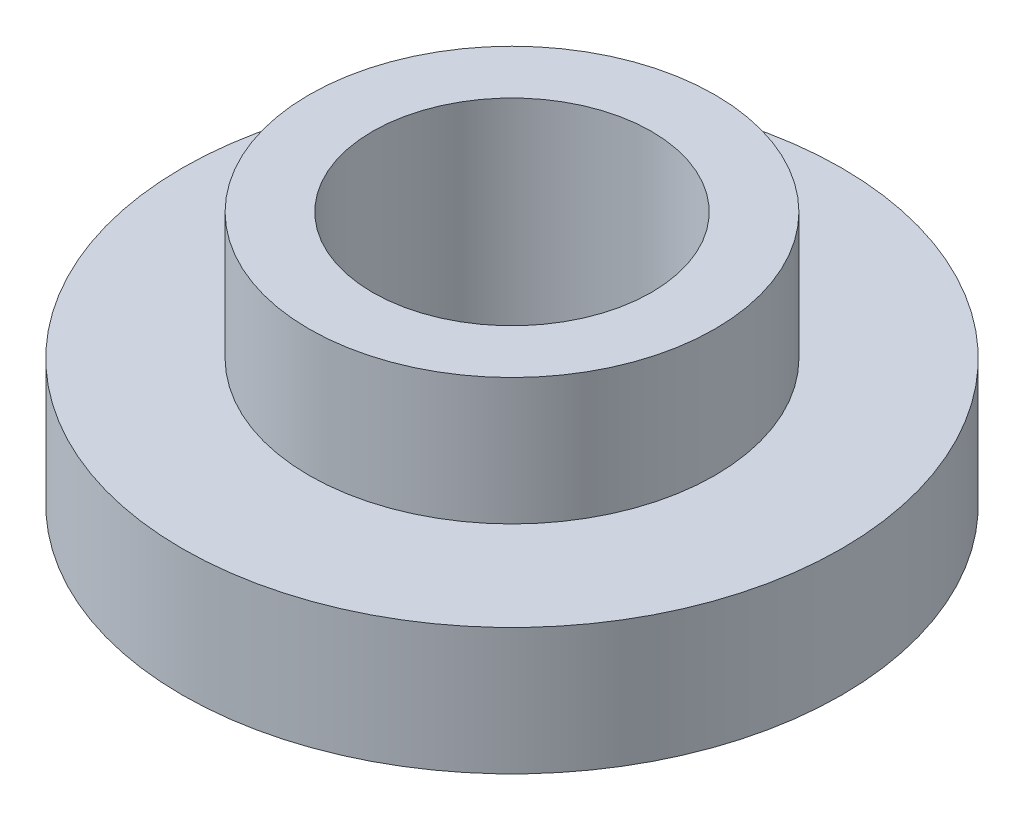
from build123d import *


with BuildPart() as part:
    # Sketch1 → Revolve1 (revolve)
    with BuildSketch(Plane.XY, mode=Mode.PRIVATE) as revolve1_sk:
        Polygon((-29.5, 0), (-65, 0), (-65, 25), (-40, 25), (-40, 50), (-27.5, 50), (-27.5, 2), align=None)
    revolve(revolve1_sk.sketch.rotate(Axis((0, 0, 0), (0, 1, 0)), 270), axis=Axis((0, 0, 0), (0, 1, 0)))


solid = part.part
